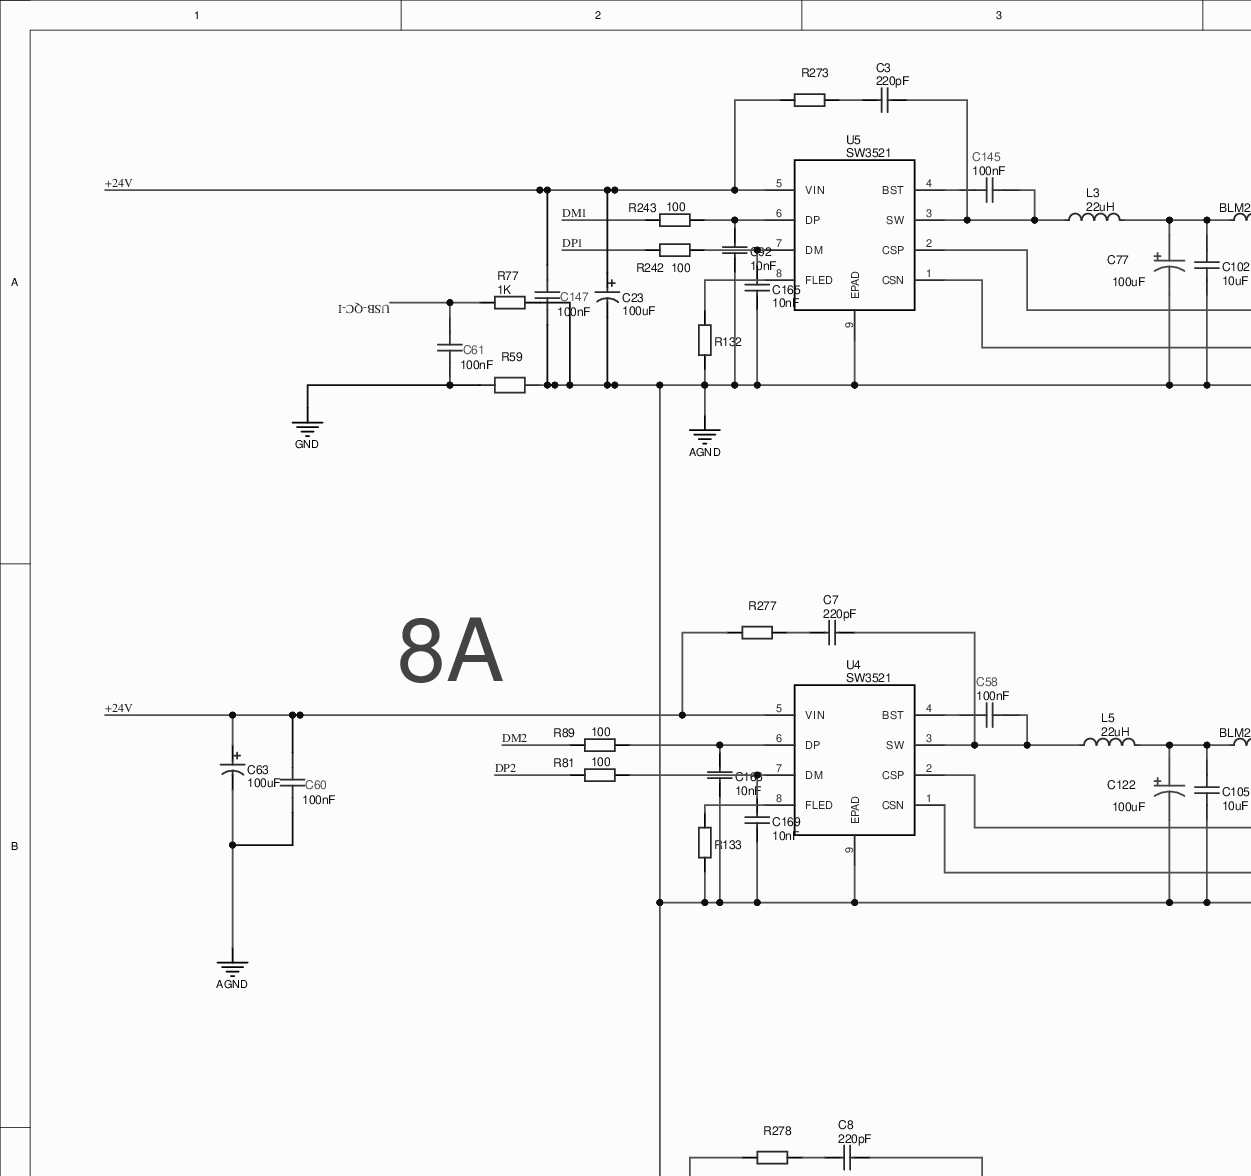
[diagram p0: MISC84402-6.SchDoc, top left]
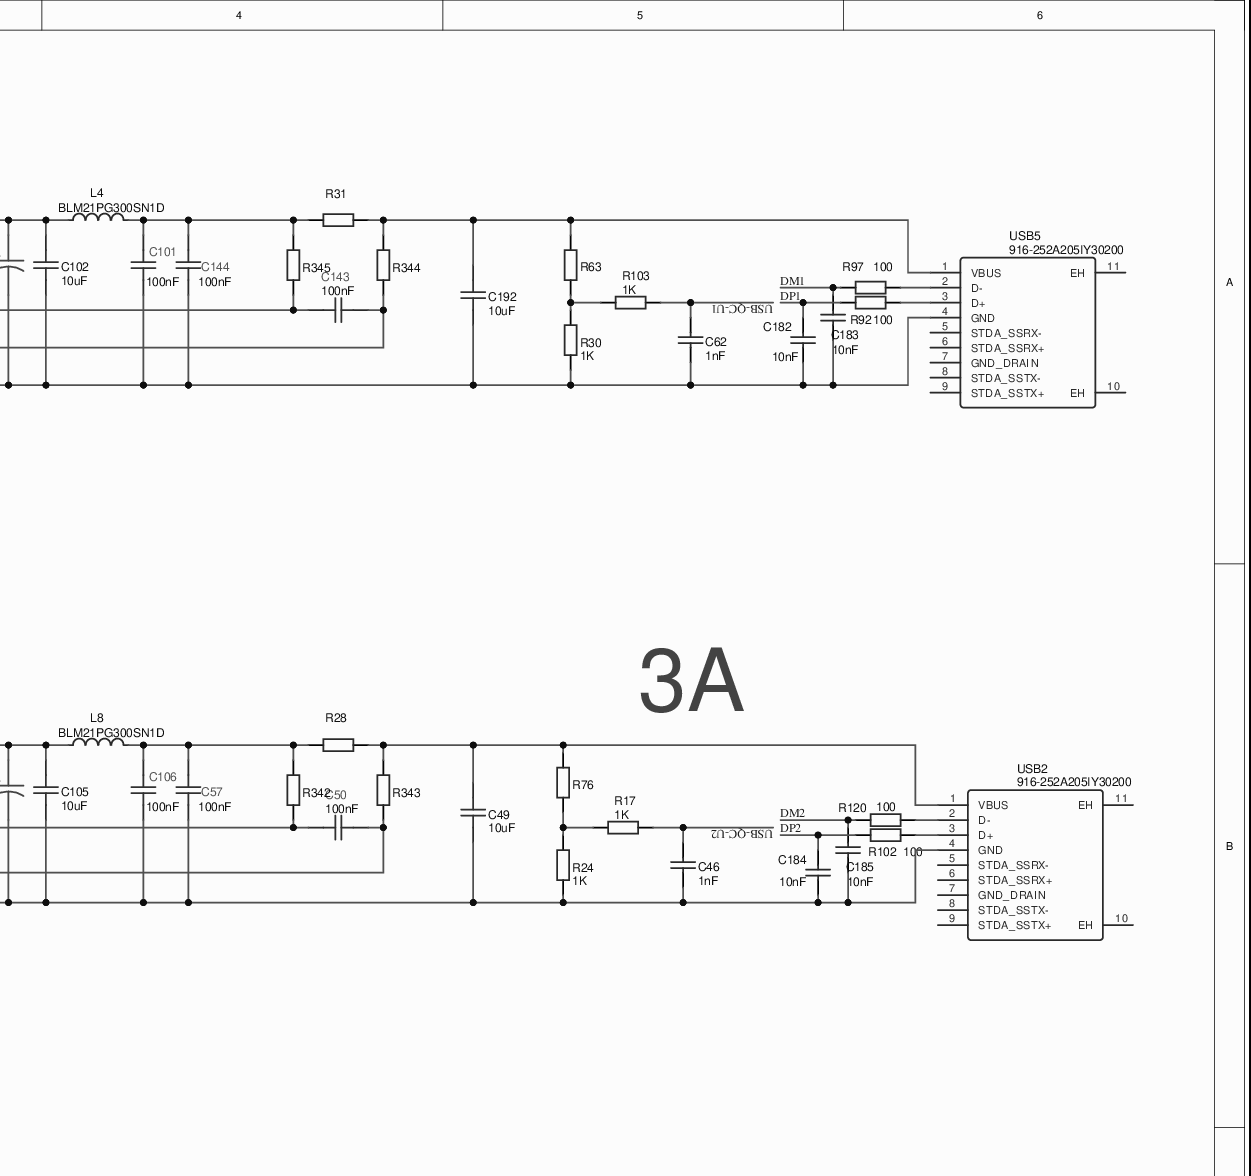
[diagram p1: MISC84402-6.SchDoc, top right]
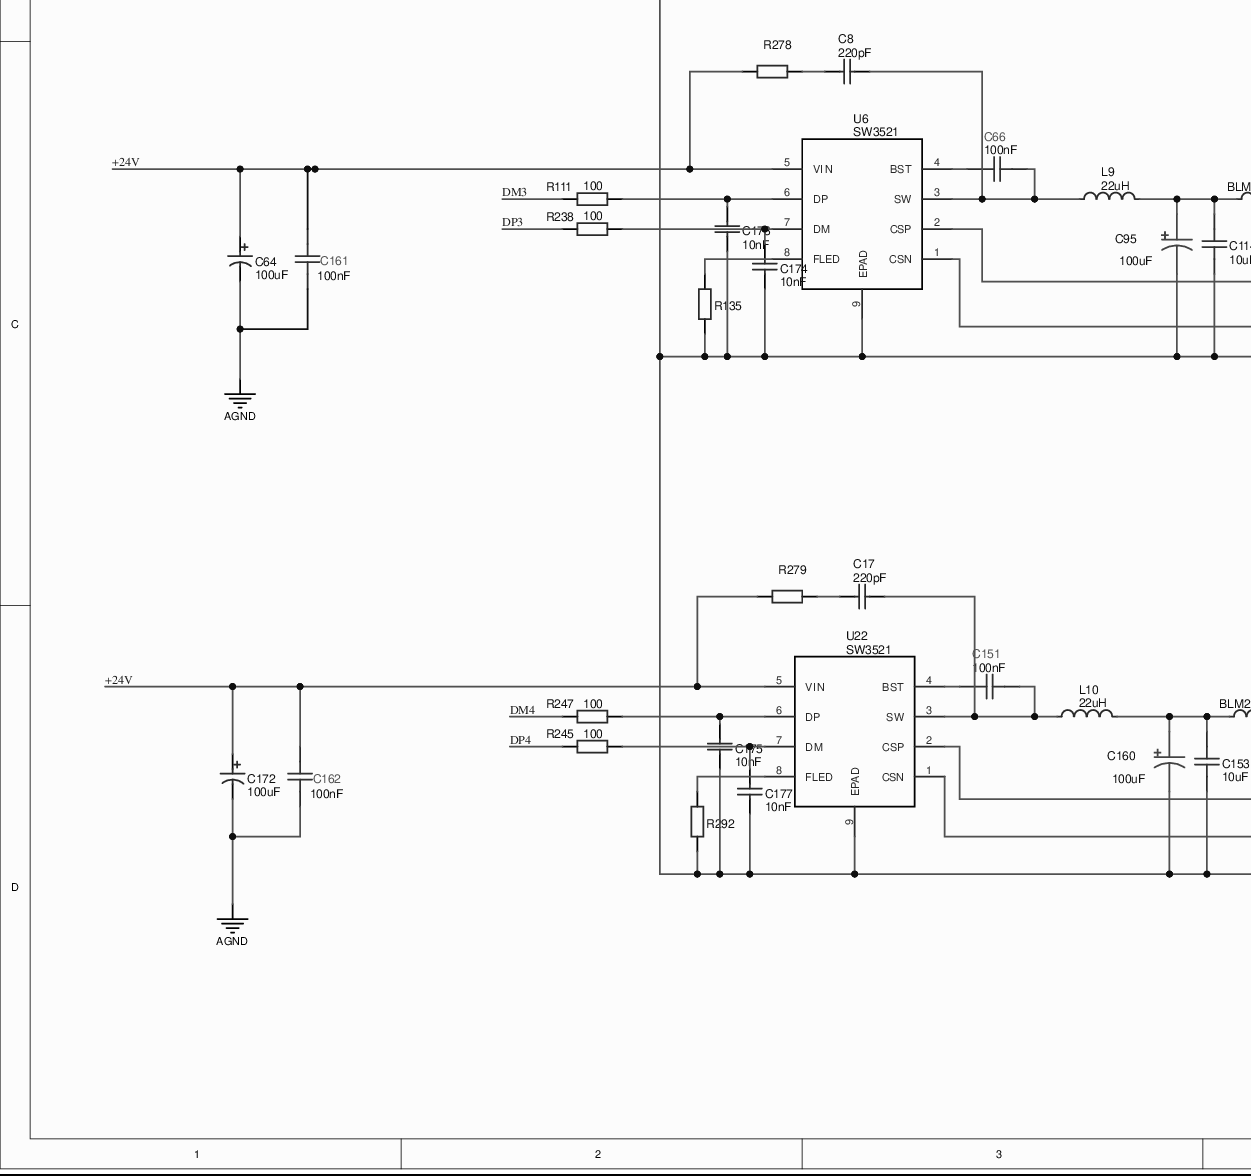
[diagram p2: MISC84402-6.SchDoc, bottom left]
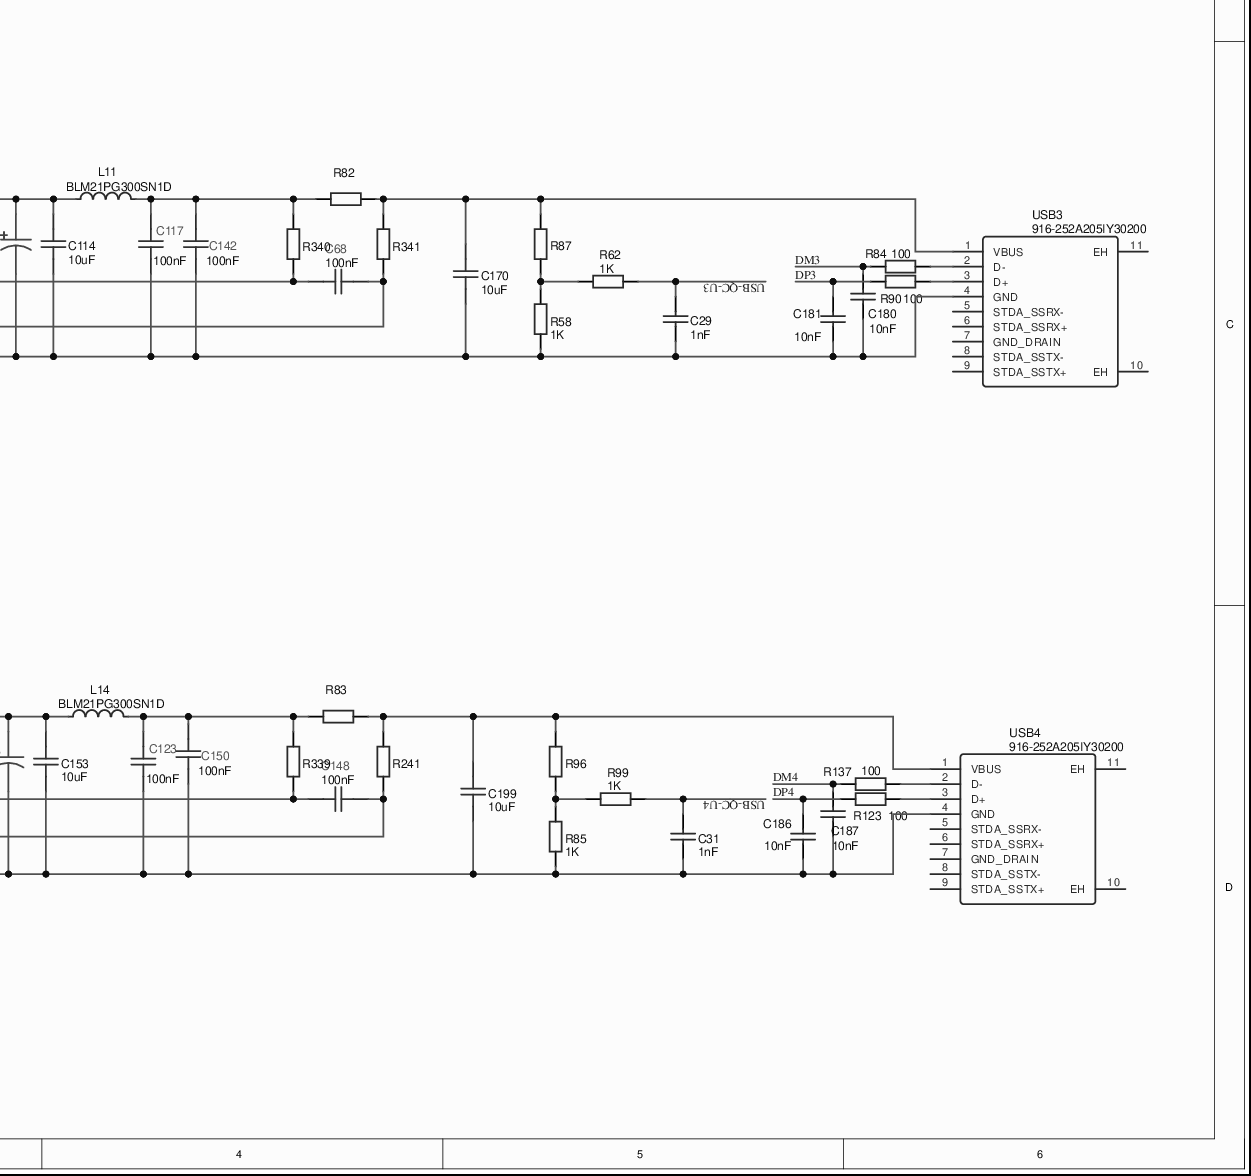
[diagram p3: MISC84402-6.SchDoc, bottom right]
# Altium project MISC84402-4.PrjPcb (part 6 of 7)

## Sheet MISC84402-6.SchDoc
size 407 x 381 mm

### Parts
C3  220pF  [C0603]
C7  220pF  [C0603]
C8  220pF  [C0603]
C17  220pF  [C0603]
C23  100uF  [CAP-SMD_BD6.3-L6.6-W6.6-FD]
C29  1nF  [C0603]
C31  1nF  [C0603]
C46  1nF  [C0603]
C49  10uF  [C0603]
C50  100nF  [C0603]
C57  100nF  [C0603]
C58  100nF  [C0603]
C60  100nF  [C0603]
C61  100nF  [C0603]
C62  1nF  [C0603]
C63  100uF  [CAP-SMD_BD6.3-L6.6-W6.6-FD]
C64  100uF  [CAP-SMD_BD6.3-L6.6-W6.6-FD]
C66  100nF  [C0603]
C68  100nF  [C0603]
C77  100uF  [CAP-SMD_BD6.3-L6.6-W6.6-FD]
C92  10nF  [C0603]
C95  100uF  [CAP-SMD_BD6.3-L6.6-W6.6-FD]
C101  100nF  [C0603]
C102  10uF  [C0603]
C105  10uF  [C0603]
C106  100nF  [C0603]
C114  10uF  [C0603]
C117  100nF  [C0603]
C122  100uF  [CAP-SMD_BD6.3-L6.6-W6.6-FD]
C123  100nF  [C0603]
C142  100nF  [C0603]
C143  100nF  [C0603]
C144  100nF  [C0603]
C145  100nF  [C0603]
C147  100nF  [C0603]
C148  100nF  [C0603]
C150  100nF  [C0603]
C151  100nF  [C0603]
C153  10uF  [C0603]
C160  100uF  [CAP-SMD_BD6.3-L6.6-W6.6-FD]
C161  100nF  [C0603]
C162  100nF  [C0603]
C165  10nF  [C0603]
C166  10nF  [C0603]
C169  10nF  [C0603]
C170  10uF  [C0603]
C172  100uF  [CAP-SMD_BD6.3-L6.6-W6.6-FD]
C173  10nF  [C0603]
C174  10nF  [C0603]
C175  10nF  [C0603]
C177  10nF  [C0603]
C180  10nF  [C0603]
C181  10nF  [C0603]
C182  10nF  [C0603]
C183  10nF  [C0603]
C184  10nF  [C0603]
C185  10nF  [C0603]
C186  10nF  [C0603]
C187  10nF  [C0603]
C192  10uF  [C0603]
C199  10uF  [C0603]
L3  22uH  [IND-SMD_L7.1-W6.8]
L4  BLM21PG300SN1D  [L0805]
L5  22uH  [IND-SMD_L7.1-W6.8]
L8  BLM21PG300SN1D  [L0805]
L9  22uH  [IND-SMD_L7.1-W6.8]
L10  22uH  [IND-SMD_L7.1-W6.8]
L11  BLM21PG300SN1D  [L0805]
L14  BLM21PG300SN1D  [L0805]
R17  1K  [R0603]
R24  1K  [R0603]
R28  (no value)  [R2512]
R30  1K  [R0603]
R31  (no value)  [R2512]
R58  1K  [R0603]
R59  (no value)  [R2512]
R62  1K  [R0603]
R63  (no value)  [R0603]
R76  (no value)  [R0603]
R77  1K  [R0603]
R81  100  [R0603]
R82  (no value)  [R2512]
R83  (no value)  [R2512]
R84  100  [R0603]
R85  1K  [R0603]
R87  (no value)  [R0603]
R89  100  [R0603]
R90  100  [R0603]
R92  100  [R0603]
R96  (no value)  [R0603]
R97  100  [R0603]
R99  1K  [R0603]
R102  100  [R0603]
R103  1K  [R0603]
R111  100  [R0603]
R120  100  [R0603]
R123  100  [R0603]
R132  (no value)  [R0603]
R133  (no value)  [R0603]
R135  (no value)  [R0603]
R137  100  [R0603]
R238  100  [R0603]
R241  (no value)  [R0603]
R242  100  [R0603]
R243  100  [R0603]
R245  100  [R0603]
R247  100  [R0603]
R273  (no value)  [R0603]
R277  (no value)  [R0603]
R278  (no value)  [R0603]
R279  (no value)  [R0603]
R292  (no value)  [R0603]
R339  (no value)  [R0603]
R340  (no value)  [R0603]
R341  (no value)  [R0603]
R342  (no value)  [R0603]
R343  (no value)  [R0603]
R344  (no value)  [R0603]
R345  (no value)  [R0603]
U4  SW3521  [ESOP-8_L4.9-W3.9-P1.27-LS6.0-BL-EP]
U5  SW3521  [ESOP-8_L4.9-W3.9-P1.27-LS6.0-BL-EP]
U6  SW3521  [ESOP-8_L4.9-W3.9-P1.27-LS6.0-BL-EP]
U22  SW3521  [ESOP-8_L4.9-W3.9-P1.27-LS6.0-BL-EP]
USB2  916-252A205IY30200  [USB-A-TH_916-252A205IY30200]
USB3  916-252A205IY30200  [USB-A-TH_916-252A205IY30200]
USB4  916-252A205IY30200  [USB-A-TH_916-252A205IY30200]
USB5  916-252A205IY30200  [USB-A-TH_916-252A205IY30200]

### Nets
AGND: C23.2 C29.1 C31.1 C46.1 C49.1 C57.1 C60.1 C62.1 C63.2 C64.2 C77.2 C92.1 C95.2 C101.1 C102.1 C105.1 C106.1 C114.1 C117.1 C122.2 C123.1 C142.1 C144.1 C147.1 C150.1 C153.1 C160.2 C161.1 C162.1 C165.1 C166.1 C169.1 C170.1 C172.2 C173.1 C174.1 C175.1 C177.1 C180.1 C181.1 C182.1 C183.1 C184.1 C185.1 C186.1 C187.1 C192.1 C199.1 R24.1 R30.1 R58.1 R59.2 R77.2 R85.1 R132.1 R133.1 R135.1 R292.1 U4.9(EPAD) U5.9(EPAD) U6.9(EPAD) U22.9(EPAD) USB2.4(GND) USB3.4(GND) USB4.4(GND) USB5.4(GND)
GND: C61.1 R59.1
+24V: C23.1 C60.2 C63.1 C64.1 C147.2 C161.2 C162.2 C172.1 R273.1 R277.1 R278.1 R279.1 U4.5(VIN) U5.5(VIN) U6.5(VIN) U22.5(VIN)
DM1: C183.2 R97.1 R243.1
DM2: C185.2 R89.1 R120.1
DM3: C180.2 R84.1 R111.1
DM4: C187.2 R137.1 R247.1
DP1: C182.2 R92.1 R242.1
DP2: C184.2 R81.1 R102.1
DP3: C181.2 R90.1 R238.1
DP4: C186.2 R123.1 R245.1
USB-QC-I: C61.2 R77.1
USB-QC-U1: C62.2 R103.2
USB-QC-U2: C46.2 R17.2
USB-QC-U3: C29.2 R62.2
USB-QC-U4: C31.2 R99.2
NetC3_1: C3.1 R273.2
NetC3_2: C3.2 C145.1 L3.1 U5.3(SW)
NetC7_1: C7.1 R277.2
NetC7_2: C7.2 C58.1 L5.1 U4.3(SW)
NetC8_1: C8.1 R278.2
NetC8_2: C8.2 C66.1 L9.1 U6.3(SW)
NetC17_1: C17.1 R279.2
NetC17_2: C17.2 C151.1 L10.1 U22.3(SW)
NetC49_2: C49.2 R28.1 R76.1 R343.1 USB2.1(VBUS)
NetC50_1: C50.1 R343.2 U4.1(CSN)
NetC50_2: C50.2 R342.2 U4.2(CSP)
NetC57_2: C57.2 C106.2 L8.2 R28.2 R342.1
NetC58_2: C58.2 U4.4(BST)
NetC66_2: C66.2 U6.4(BST)
NetC68_1: C68.1 R341.2 U6.1(CSN)
NetC68_2: C68.2 R340.2 U6.2(CSP)
NetC77_1: C77.1 C102.2 L3.2 L4.1
NetC92_2: C92.2 R243.2 U5.6(DP)
NetC95_1: C95.1 C114.2 L9.2 L11.1
NetC101_2: C101.2 C144.2 L4.2 R31.2 R345.1
NetC105_2: C105.2 C122.1 L5.2 L8.1
NetC117_2: C117.2 C142.2 L11.2 R82.2 R340.1
NetC123_2: C123.2 C150.2 L14.2 R83.2 R339.1
NetC143_1: C143.1 R344.2 U5.1(CSN)
NetC143_2: C143.2 R345.2 U5.2(CSP)
NetC145_2: C145.2 U5.4(BST)
NetC148_1: C148.1 R241.2 U22.1(CSN)
NetC148_2: C148.2 R339.2 U22.2(CSP)
NetC151_2: C151.2 U22.4(BST)
NetC153_2: C153.2 C160.1 L10.2 L14.1
NetC165_2: C165.2 R242.2 U5.7(DM)
NetC166_2: C166.2 R89.2 U4.6(DP)
NetC169_2: C169.2 R81.2 U4.7(DM)
NetC170_2: C170.2 R82.1 R87.1 R341.1 USB3.1(VBUS)
NetC173_2: C173.2 R111.2 U6.6(DP)
NetC174_2: C174.2 R238.2 U6.7(DM)
NetC175_2: C175.2 R247.2 U22.6(DP)
NetC177_2: C177.2 R245.2 U22.7(DM)
NetC192_2: C192.2 R31.1 R63.1 R344.1 USB5.1(VBUS)
NetC199_2: C199.2 R83.1 R96.1 R241.1 USB4.1(VBUS)
NetR17_1: R17.1 R24.2 R76.2
NetR30_2: R30.2 R63.2 R103.1
NetR58_2: R58.2 R62.1 R87.2
NetR84_2: R84.2 USB3.2(D-)
NetR85_2: R85.2 R96.2 R99.1
NetR90_2: R90.2 USB3.3(D+)
NetR92_2: R92.2 USB5.3(D+)
NetR97_2: R97.2 USB5.2(D-)
NetR102_2: R102.2 USB2.3(D+)
NetR120_2: R120.2 USB2.2(D-)
NetR123_2: R123.2 USB4.3(D+)
NetR132_2: R132.2 U5.8(FLED)
NetR133_2: R133.2 U4.8(FLED)
NetR135_2: R135.2 U6.8(FLED)
NetR137_2: R137.2 USB4.2(D-)
NetR292_2: R292.2 U22.8(FLED)

Not connected (* = marked no-connect by the designer): USB2 5(STDA_SSRX-) 6(STDA_SSRX+) 7(GND_DRAIN) 8(STDA_SSTX-) 9(STDA_SSTX+) 10(EH) 11(EH); USB3 5(STDA_SSRX-) 6(STDA_SSRX+) 7(GND_DRAIN) 8(STDA_SSTX-) 9(STDA_SSTX+) 10(EH) 11(EH); USB4 5(STDA_SSRX-) 6(STDA_SSRX+) 7(GND_DRAIN) 8(STDA_SSTX-) 9(STDA_SSTX+) 10(EH) 11(EH); USB5 5(STDA_SSRX-) 6(STDA_SSRX+) 7(GND_DRAIN) 8(STDA_SSTX-) 9(STDA_SSTX+) 10(EH) 11(EH)

### Notes on the sheet
- 8A
- 3A

### Library data of the parts
C3 C7 C8 C17 = 220pF: BOM_Manufacturer Part: CL10B221KB8NNNC; BOM_Manufacturer: SAMSUNG; nameAlias: Capacitance; BOM_Supplier: LCSC; BOM_Supplier Part: C1603; BOM_JLCPCB Part Class: Basic Part; spicePre: C; spiceSymbolName: CL10B221KB8NNNC
C23 C63 C64 C172 = 100uF: BOM_Manufacturer: ROQANG; BOM_Manufacturer Part: RT1V101M0607; nameAlias: Capacitance; Contributor: LCSC; BOM_Supplier: LCSC; BOM_Supplier Part: C267470; BOM_JLCPCB Part Class: Extended Part; spicePre: C; spiceSymbolName: RT1V101M0607
C29 C31 C46 C62 = 1nF: BOM_Manufacturer Part: CL10B102KB8NNNC; BOM_Manufacturer: SAMSUNG; nameAlias: Capacitance; BOM_Supplier: LCSC; BOM_Supplier Part: C1588; BOM_JLCPCB Part Class: Basic Part; spicePre: C; spiceSymbolName: CL10B102KB8NNNC
C49 C102 C105 C114 C153 C170 C192 C199 = 10uF: BOM_Manufacturer: FH(Guangdong Fenghua Advanced Tech); BOM_Manufacturer Part: 0603X106M250NT; nameAlias: Capacitance; Contributor: LCSC; BOM_Supplier: LCSC; BOM_Supplier Part: C479655; BOM_JLCPCB Part Class: Extended Part; spicePre: C; spiceSymbolName: 0603X106M250NT
C50 C57 C58 C60 C61 C66 C68 C101 C106 C117 C123 C142-C145 C147 C148 C150 C151 C161 C162 = 100nF: BOM_Manufacturer: SAMSUNG; BOM_Manufacturer Part: CL10B104KC8NNNC; nameAlias: Capacitance; BOM_Supplier: LCSC; BOM_Supplier Part: C15725; BOM_JLCPCB Part Class: Extended Part; spicePre: C; spiceSymbolName: CL10B104KC8NNNC
C77 C95 C122 C160 = 100uF: BOM_Manufacturer: Lelon; BOM_Manufacturer Part: HBW101M1ETR-0608; nameAlias: Capacitance; Contributor: LCSC; BOM_Supplier: LCSC; BOM_Supplier Part: C311671; BOM_JLCPCB Part Class: Extended Part; spicePre: C; spiceSymbolName: HBW101M1ETR-0608
C92 C165 C166 C169 C173-C175 C177 C180-C187 = 10nF: BOM_Manufacturer: YAGEO; BOM_Manufacturer Part: CC0603KRX7R9BB103; nameAlias: Capacitance; BOM_Supplier: LCSC; BOM_Supplier Part: C100042; BOM_JLCPCB Part Class: Extended Part; spicePre: C; spiceSymbolName: CC0603KRX7R9BB103
L3 L5 L9 L10 = 22uH: BOM_Manufacturer: Bao Cheng Elec; BOM_Manufacturer Part: BCIHP0730-6R8M; nameAlias: Inductance; Contributor: LCSC; BOM_Supplier: LCSC; BOM_Supplier Part: C237912; BOM_JLCPCB Part Class: Extended Part; spicePre: L; spiceSymbolName: BCIHP0730-6R8M
L4 L8 L11 L14 = BLM21PG300SN1D: BOM_Manufacturer: MuRata; nameAlias: Value(H); BOM_Supplier: LCSC; BOM_Manufacturer Part: BLM21PG300SN1D; BOM_Supplier Part: C16903; BOM_JLCPCB Part Class: Extended Part; spicePre: L; spiceSymbolName: BLM21PG300SN1D
R17 R24 R30 R58 R62 R77 R85 R99 R103 = 1K: BOM_Manufacturer: FH; BOM_Manufacturer Part: RS-03K102JT; nameAlias: Resistance (Ohms); BOM_Supplier: LCSC; BOM_Supplier Part: C73797; spicePre: R; spiceSymbolName: RS-03K102JT
R28 R31 R82 R83 = (no symbol name): BOM_Manufacturer Part: MRF6432(2512)LR010JTS; BOM_Manufacturer: SUP; BOM_Supplier Part: C76272; BOM_Supplier: LCSC; BOM_JLCPCB Part Class: Extended Part; spicePre: R; spiceSymbolName: MRF6432(2512)LR010JTS
R59 = (no symbol name): BOM_Manufacturer: Milliohm; BOM_Manufacturer Part: GX2512-2W-20mR-1%; Resistance (Ohms): 0.02; nameAlias: Resistance; Contributor: LCSC; BOM_Supplier: LCSC; BOM_Supplier Part: C500720; BOM_JLCPCB Part Class: Extended Part; spicePre: R; spiceSymbolName: GX2512-2W-20MR-1%
R63 R76 R87 R96 R132 R133 R135 R292 = (no symbol name): BOM_Manufacturer: UniOhm; BOM_Manufacturer Part: 0603WAF1002T5E; nameAlias: Resistance; Resistance (Ohms): 10K; BOM_Supplier: LCSC; BOM_Supplier Part: C25804; BOM_JLCPCB Part Class: Basic Part; spicePre: R; spiceSymbolName: 0603WAF1002T5E
R81 R84 R89 R90 R92 R97 R102 R111 R120 R123 R137 R238 R242 R243 R245 R247 = 100: BOM_Manufacturer: YAGEO; BOM_Manufacturer Part: RC0603FR-07100RL; nameAlias: Resistance (Ohms); BOM_Supplier: LCSC; BOM_Supplier Part: C105588; BOM_JLCPCB Part Class: Extended Part; spicePre: R; spiceSymbolName: RC0603FR-07100RL
R241 R339-R345 = (no symbol name): BOM_Manufacturer: UniOhm; BOM_Manufacturer Part: 0603WAF100KT5E; nameAlias: Resistance; Resistance (Ohms): 1; BOM_Supplier: LCSC; BOM_Supplier Part: C22936; BOM_JLCPCB Part Class: Basic Part; spicePre: R; spiceSymbolName: 0603WAF100KT5E
R273 R277-R279 = (no symbol name): BOM_Manufacturer: UniOhm; BOM_Manufacturer Part: 0603WAF470KT5E; nameAlias: Resistance; Resistance (Ohms): 4.7; BOM_Supplier: LCSC; BOM_Supplier Part: C23164; BOM_JLCPCB Part Class: Basic Part; spicePre: R; spiceSymbolName: 0603WAF470KT5E
U4-U6 U22 = SW3521: BOM_Manufacturer: iSmartWare; Contributor: Levepan; BOM_Manufacturer Part: SW3521; link: http://www.ismartware.com/info/85.html; spicePre: U; spiceSymbolName: SW3521
USB2-USB5 = 916-252A205IY30200: Contributor: LCSC; BOM_Supplier: LCSC; BOM_Supplier Part: C2763053; BOM_Manufacturer Part: 916-252A205IY30200; JLCPCB Part Class: Extended Part; spicePre: U; spiceSymbolName: 916-252A205IY30200